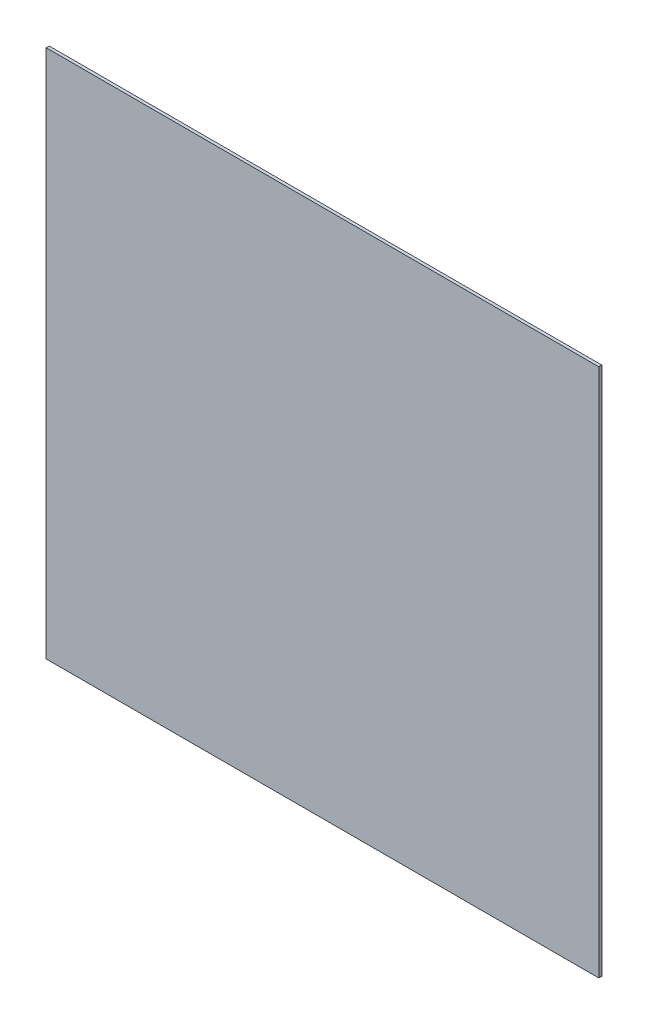
from build123d import *

# Parameters (mm, degrees)
SKETCH_1_W      = 926
SKETCH_1_H      = 887
EXTRUDE_1_DEPTH = 5


with BuildPart() as part:
    # 草图1 → 凸台-拉伸1 (new body)
    with BuildSketch(Plane.XY):
        Rectangle(SKETCH_1_W, SKETCH_1_H)
    extrude(amount=EXTRUDE_1_DEPTH)


solid = part.part
